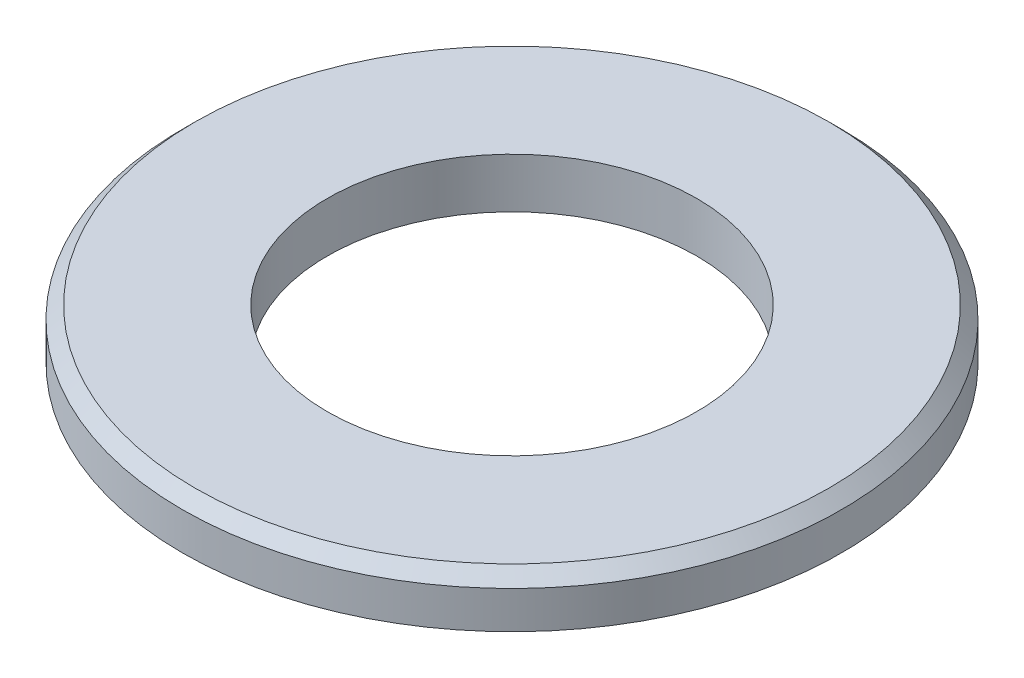
SolidWorks part; units mm, degrees
ref_plane "基准面1" through (0, 0, 0) normal (0, 0, 1) x (1, 0, 0)
ref_plane "基准面2" through (0, 0, 0) normal (0, 1, 0) x (1, 0, 0)
ref_plane "基准面3" through (0, 0, 0) normal (1, 0, 0) x (0, 0, -1)
sketch "尺寸草图" plane through (0, 0, 0) normal (0, 0, 1) x (1, 0, 0)
  line L0 (0, 0) -> (9.1, 0)
  point P3 (5, 0)
  point P4 (66, 0)
  point P5 (37, 0)
sketch "草图1" plane through (0, 0, 0) normal (0, 0, 1) x (1, 0, 0)
  line L0 (0, 0) -> (0, 52.7318) construction
  line L1 (-31.75, 13.6445) -> (-33, 12.3945)
  line L2 (-18.5, 8.6445) -> (-33, 8.6445)
  line L3 (-18.5, 8.6445) -> (-18.5, 13.6445)
  line L4 (-18.5, 13.6445) -> (-31.75, 13.6445)
  line L5 (-33, 8.6445) -> (-33, 12.3945)
  point P4 (-33, 13.6445)
revolve "基体-旋转" add sketch "草图1" angle 360 about L0
equation "\"h@草图1\" = \"h@尺寸草图\""
equation "\"D1@草图1\" = \"d1@尺寸草图\" / 2"
equation "\"D2@草图1\" = \"d2@尺寸草图\" / 2"
equation "\"D5@草图1\" = \"h@草图1\" *0.25"
